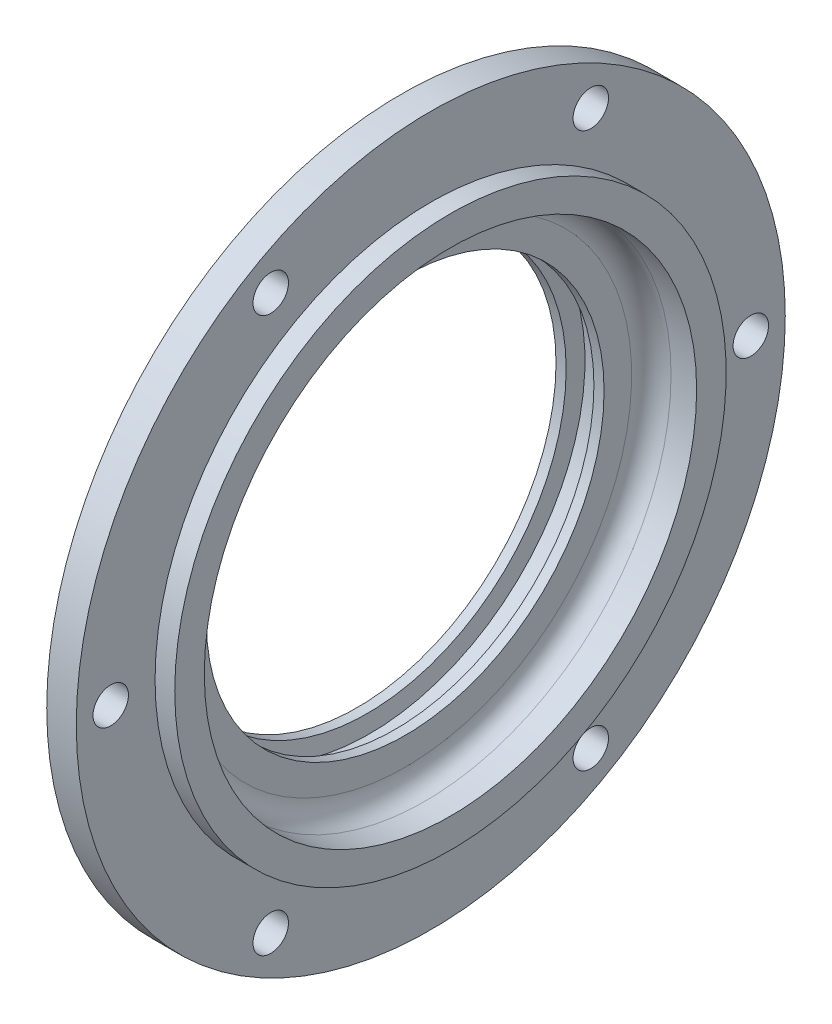
SolidWorks part; units mm, degrees
material "Q235"
ref_plane "Front Plane" through (0, 0, 0) normal (0, 0, 1) x (1, 0, 0)
ref_plane "Top Plane" through (0, 0, 0) normal (0, 1, 0) x (1, 0, 0)
ref_plane "Right Plane" through (0, 0, 0) normal (1, 0, 0) x (0, 0, -1)
sketch "Sketch1" plane through (0, 0, 0) normal (0, 1, 0) x (1, 0, 0)
  line L0 (9248.1354, 152.4737) -> (9238.1354, 152.4737)
  line L1 (9238.1354, 152.4737) -> (9238.1354, 192.4737)
  line L2 (9223.1354, 192.4737) -> (9223.1354, 162.4737)
  line L3 (9248.1354, 152.4737) -> (9248.1354, 137.4737)
  line L4 (9238.1354, 152.4737) -> (9248.1354, 152.4737)
  line L5 (9213.1354, 152.4737) -> (9210.7354, 152.4737)
  line L6 (9235.1354, 137.4737) -> (9248.1354, 137.4737)
  line L7 (9225.1354, 127.4737) -> (9225.1354, 113.4737)
  line L8 (9206.9354, 121.9737) -> (9218.9354, 121.9737)
  line L9 (9218.9354, 121.9737) -> (9219.9791, 113.4737)
  line L10 (9206.9354, 121.9737) -> (9205.8918, 113.4737)
  line L11 (9200.7354, 142.4737) -> (9200.7354, 113.4737)
  line L12 (9200.7354, 113.4737) -> (9205.8918, 113.4737)
  line L13 (9219.9791, 113.4737) -> (9225.1354, 113.4737)
  line L14 (9238.1354, 152.4737) -> (9248.1354, 152.4737)
  line L15 (9223.1354, 192.4737) -> (9238.1354, 192.4737)
  line L16 (9092.8699, 12.4737) -> (9332.1207, 12.4737) construction
  line L17 (9092.8699, 113.4737) -> (9332.1207, 113.4737) construction
  arc A0 (9210.7354, 152.4737) -> (9200.7354, 142.4737) centre (9210.7354, 142.4737) ccw
  arc A1 (9213.1354, 152.4737) -> (9223.1354, 162.4737) centre (9213.1354, 162.4737) ccw
  arc A2 (9235.1354, 137.4737) -> (9225.1354, 127.4737) centre (9235.1354, 127.4737) ccw
  dimension "D1" = 125
  dimension "D2" = 14
  dimension "D3" = 180
  dimension "D4" = 30
  dimension "D5" = 15
  dimension "D6" = 40
  dimension "D7" = 15
  dimension "D8" = 24.4
  dimension "D9" = 101
revolve "Revolve1" add sketch "Sketch1" angle 360 about L16
sketch "Sketch2" plane through (9238.1354, 0, 0) normal (1, 0, 0) x (0, 0, -1)
  line L0 (12.4737, 0) -> (12.4737, 193.77) construction
  line L1 (12.4737, 0) -> (-96.8977, 189.437) construction
  circle A0 centre (12.4737, 0) radius 162.5 construction
  circle A1 centre (-68.7763, 140.7291) radius 9
  circle A2 centre (93.7237, 140.7291) radius 9
  circle A3 centre (174.9737, 0) radius 9
  circle A4 centre (93.7237, -140.7291) radius 9
  circle A5 centre (-68.7763, -140.7291) radius 9
  circle A6 centre (-150.0263, 0) radius 9
  point P19 (12.4737, 0)
  dimension "D1" = 6
  dimension "D2" = 30
extrude "Cut-Extrude1" cut sketch "Sketch2" against normal through all
